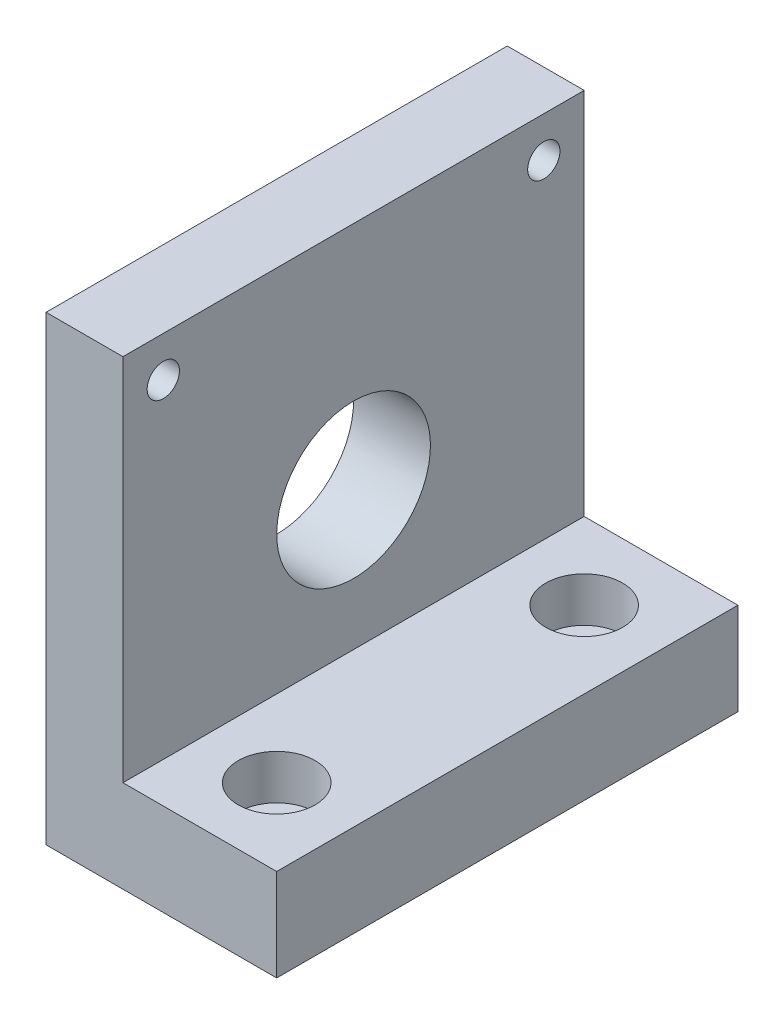
from build123d import *

# Parameters (mm, degrees)
EXTRUDE_1_DEPTH     = 60
SKETCH_2_R          = 10
CUT_EXTRUDE_1_DEPTH = 78.808619714
SKETCH_3_R          = 2.1
CUT_EXTRUDE_2_DEPTH = 78.808619714
SKETCH_4_R          = 2.75
CUT_EXTRUDE_3_DEPTH = 81.17516917
SKETCH_5_R          = 5
CUT_EXTRUDE_4_DEPTH = 5.8


with BuildPart() as part:
    # 草图1 → 凸台-拉伸1 (new body)
    with BuildSketch(Plane.XY):
        Polygon((-12.892307692, 45.323076923), (-12.892307692, -2.676923077), (7.107692308, -2.676923077), (7.107692308, -14.676923077), (-22.892307692, -14.676923077), (-22.892307692, 45.323076923), align=None)
    extrude(amount=EXTRUDE_1_DEPTH)

    # 草图2 → 切除-拉伸1 (cut, through all)
    with BuildSketch(Plane(origin=(-12.892307692, 0, 0), x_dir=(0, 0, -1), z_dir=(1, 0, 0))):
        with Locations(Location((-30, 15.323076923, 0), (0, 0, 90))):
            Circle(SKETCH_2_R)
    extrude(amount=-CUT_EXTRUDE_1_DEPTH, mode=Mode.SUBTRACT)

    # 草图3 → 切除-拉伸2 (cut, through all)
    with BuildSketch(Plane(origin=(-12.892307692, 0, 0), x_dir=(0, 0, -1), z_dir=(1, 0, 0))):
        with Locations(Location((-54.75, 40.073076923, 0), (0, 0, 90))):
            Circle(SKETCH_3_R)
        with Locations(Location((-5.25, 40.073076923, 0), (0, 0, 90))):
            Circle(SKETCH_3_R)
    extrude(amount=-CUT_EXTRUDE_2_DEPTH, mode=Mode.SUBTRACT)

    # 草图4 → 切除-拉伸3 (cut, through all)
    with BuildSketch(Plane(origin=(0, -2.676923077, 0), x_dir=(1, 0, 0), z_dir=(0, 1, 0))):
        with Locations(Location((-2.892307692, -10, 0), (0, 0, 270))):
            Circle(SKETCH_4_R)
        with Locations(Location((-2.892307692, -50, 0), (0, 0, 270))):
            Circle(SKETCH_4_R)
    extrude(amount=-CUT_EXTRUDE_3_DEPTH, mode=Mode.SUBTRACT)

    # 草图5 → 切除-拉伸4 (cut)
    with BuildSketch(Plane(origin=(0, -2.676923077, 0), x_dir=(1, 0, 0), z_dir=(0, 1, 0))):
        with Locations(Location((-2.892307692, -10, 0), (0, 0, 270))):
            Circle(SKETCH_5_R)
        with Locations(Location((-2.892307692, -50, 0), (0, 0, 270))):
            Circle(SKETCH_5_R)
    extrude(amount=-CUT_EXTRUDE_4_DEPTH, mode=Mode.SUBTRACT)


solid = part.part
